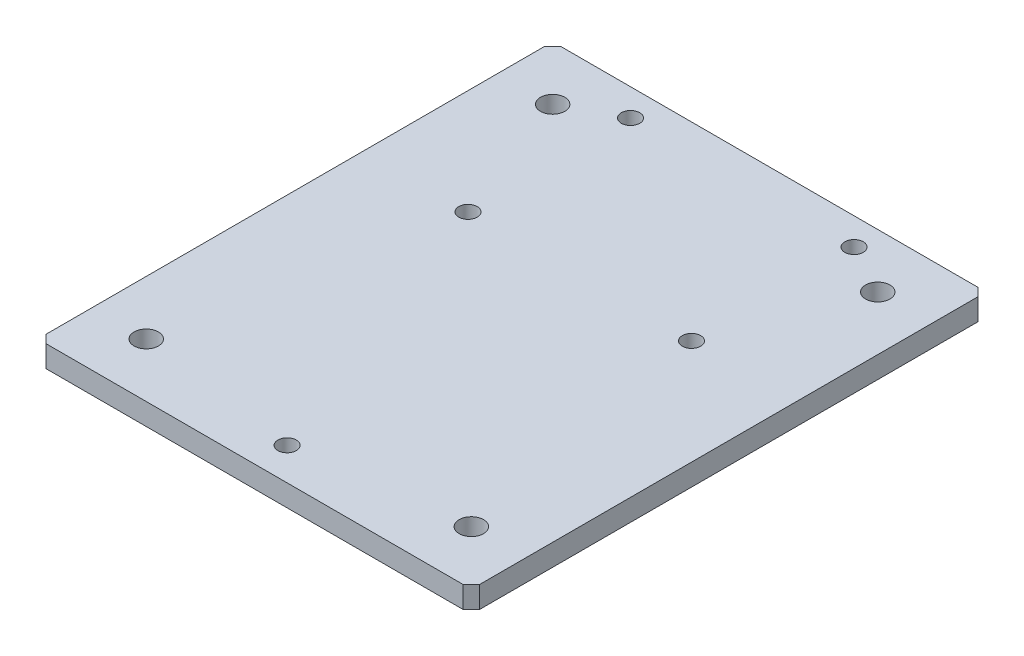
from build123d import *

# Parameters (mm, degrees)
SKETCH_1_W            = 160
SKETCH_1_H            = 190
EXTRUDE_1_DEPTH       = 4
CHAMFER_1_SIZE        = 3
HOLE_WIZARD_9_0_9_1_D = 9
HOLE_WIZARD_M8_2_D    = 6.8
HOLE_WIZARD_M8_1_D    = 6.8


with BuildPart() as part:
    # 草图1 → 凸台-拉伸1 (new, symmetric)
    with BuildSketch(Plane(origin=(0, 0, 0), x_dir=(1, 0, 0), z_dir=(0, 1, 0))):
        Rectangle(SKETCH_1_W, SKETCH_1_H)
    extrude(amount=EXTRUDE_1_DEPTH, both=True)

    # 倒角1
    chamfer_1_edges = [part.edges().sort_by_distance(p)[0] for p in [
        (80, 0, 95),
        (-80, 0, 95),
        (-80, 0, -95),
        (80, 0, -95),
    ]]
    chamfer(chamfer_1_edges, length=CHAMFER_1_SIZE)

    # Ø9.0 (9) 直径孔1 (through all)
    with Locations(Plane(origin=(0, -4, 0), x_dir=(-1, 0, 0), z_dir=(0, -1, 0))):
        with Locations((-60, -75), (60, -75), (60, 75), (-60, 75)):
            Hole(HOLE_WIZARD_9_0_9_1_D / 2)

    # M8 螺纹孔2 (through all)
    with Locations(Plane(origin=(0, -4, 0), x_dir=(-1, 0, 0), z_dir=(0, -1, 0))):
        with Locations((-41.25, 25), (-41.25, 85), (41.25, 85), (41.25, 25)):
            Hole(HOLE_WIZARD_M8_2_D / 2)

    # M8 螺纹孔1 (through all)
    with Locations(Plane(origin=(0, -4, 0), x_dir=(-1, 0, 0), z_dir=(0, -1, 0))):
        with Locations((0, -83)):
            Hole(HOLE_WIZARD_M8_1_D / 2)


solid = part.part
